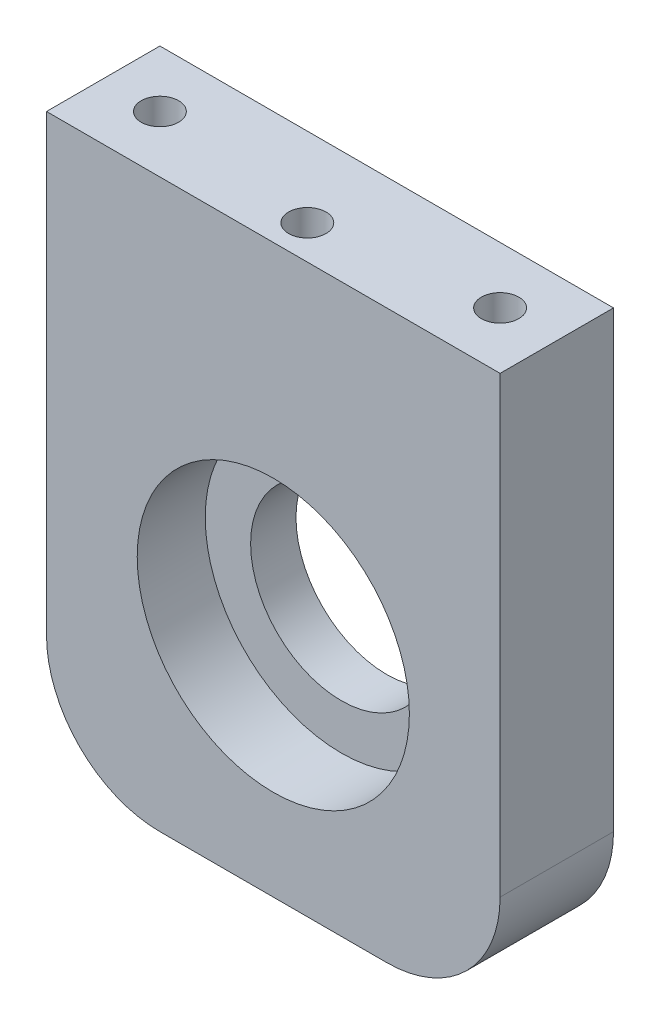
from build123d import *

# Parameters (mm, degrees)
SKETCH_1_W              = 40
SKETCH_1_H              = 50
EXTRUDE_1_DEPTH         = 10
SKETCH_2_R              = 12
CUT_EXTRUDE_1_DEPTH     = 6
SKETCH_3_R              = 8
CUT_EXTRUDE_2_DEPTH     = 33.57299495
HOLE_WIZARD_M4_1_D      = 3.3
HOLE_WIZARD_M4_1_DEPTH  = 10
HOLE_WIZARD_M4_1_TIP    = 0.991420021
FILLET_1_R              = 10
HOLE_WIZARD_M4_3_REACH  = 56.772
HOLE_WIZARD_M4_3_BORE_R = 1.65


with BuildPart() as part:
    # 草图1 → 凸台-拉伸1 (new body)
    with BuildSketch(Plane.XY):
        Rectangle(SKETCH_1_W, SKETCH_1_H)
    extrude(amount=EXTRUDE_1_DEPTH)

    # 草图2 → 切除-拉伸1 (cut)
    with BuildSketch(Plane.XY.offset(10)):
        with Locations((0, -5)):
            Circle(SKETCH_2_R)
    extrude(amount=-CUT_EXTRUDE_1_DEPTH, mode=Mode.SUBTRACT)

    # 草图3 → 切除-拉伸2 (cut, through all)
    with BuildSketch(Plane.XY.offset(4)):
        with Locations((0, -5)):
            Circle(SKETCH_3_R)
    extrude(amount=-CUT_EXTRUDE_2_DEPTH, mode=Mode.SUBTRACT)

    # M4 螺纹孔1
    with Locations(Plane(origin=(0, 25, 0), x_dir=(1, 0, 0), z_dir=(0, 1, 0))):
        with Locations((-15, -5), (15, -5)):
            Hole(HOLE_WIZARD_M4_1_D / 2, depth=HOLE_WIZARD_M4_1_DEPTH)
            with Locations((0, 0, -(HOLE_WIZARD_M4_1_DEPTH + HOLE_WIZARD_M4_1_TIP / 2))):  # 118° drill point
                Cone(0, HOLE_WIZARD_M4_1_D / 2, HOLE_WIZARD_M4_1_TIP, mode=Mode.SUBTRACT)

    # 圆角1
    fillet_1_edges = [part.edges().sort_by_distance(p)[0] for p in [
        (20, -25, 5),
        (-20, -25, 5),
    ]]
    fillet(fillet_1_edges, radius=FILLET_1_R)

    # M4 螺纹孔3 bore → M4 螺纹孔3 (cut, up to next)
    with BuildSketch(Plane(origin=(0, 25, 0), x_dir=(1, 0, 0), z_dir=(0, 1, 0)), mode=Mode.PRIVATE) as hole_wizard_m4_3_sk1:
        with Locations((0, -7)):
            Circle(HOLE_WIZARD_M4_3_BORE_R)
    hole_wizard_m4_3_tool1 = extrude(hole_wizard_m4_3_sk1.sketch, amount=-HOLE_WIZARD_M4_3_REACH, mode=Mode.PRIVATE) & part.part
    add(hole_wizard_m4_3_tool1.solids().sort_by_distance((0, 25, 7))[0], mode=Mode.SUBTRACT)


solid = part.part
